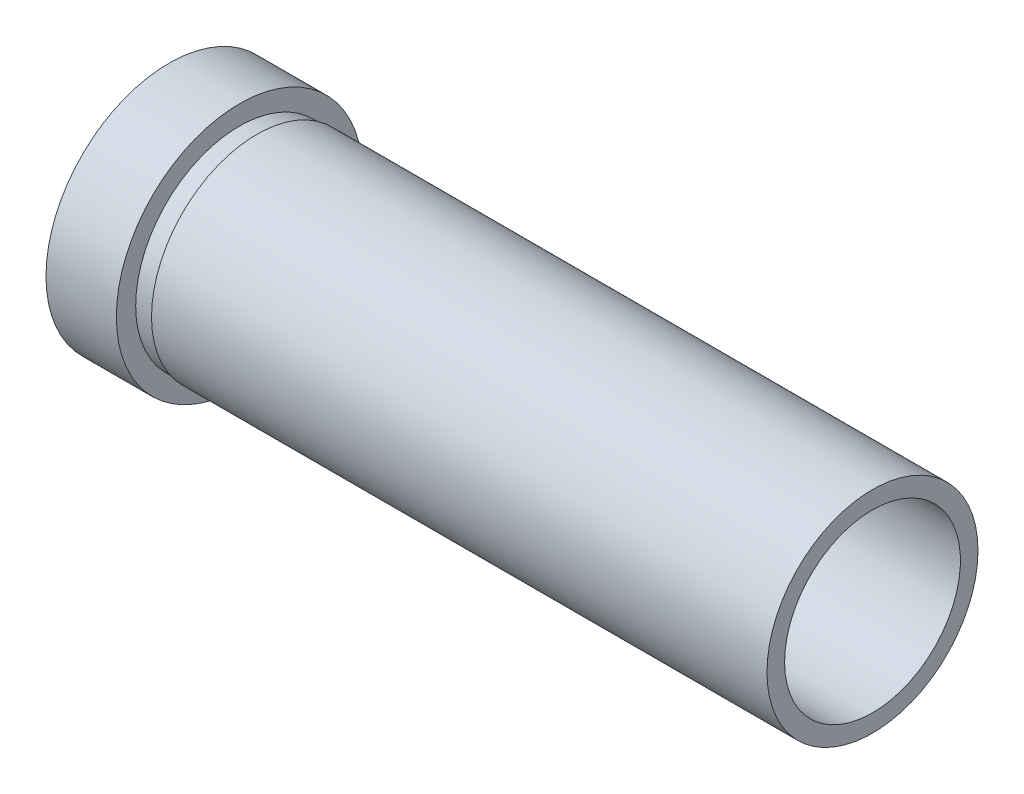
from build123d import *


with BuildPart() as part:
    # Sketch1 → Revolve1 (revolve)
    with BuildSketch(Plane.XY, mode=Mode.PRIVATE) as revolve1_sk:
        Polygon((-20, 7), (-20, 5), (20, 5), (20, 6), (-15, 6), (-15, 5.9), (-16, 5.9), (-16, 7), align=None)
    revolve(revolve1_sk.sketch.rotate(Axis((20, 0, 0), (-1, 0, 0)), 270), axis=Axis((20, 0, 0), (-1, 0, 0)))


solid = part.part
